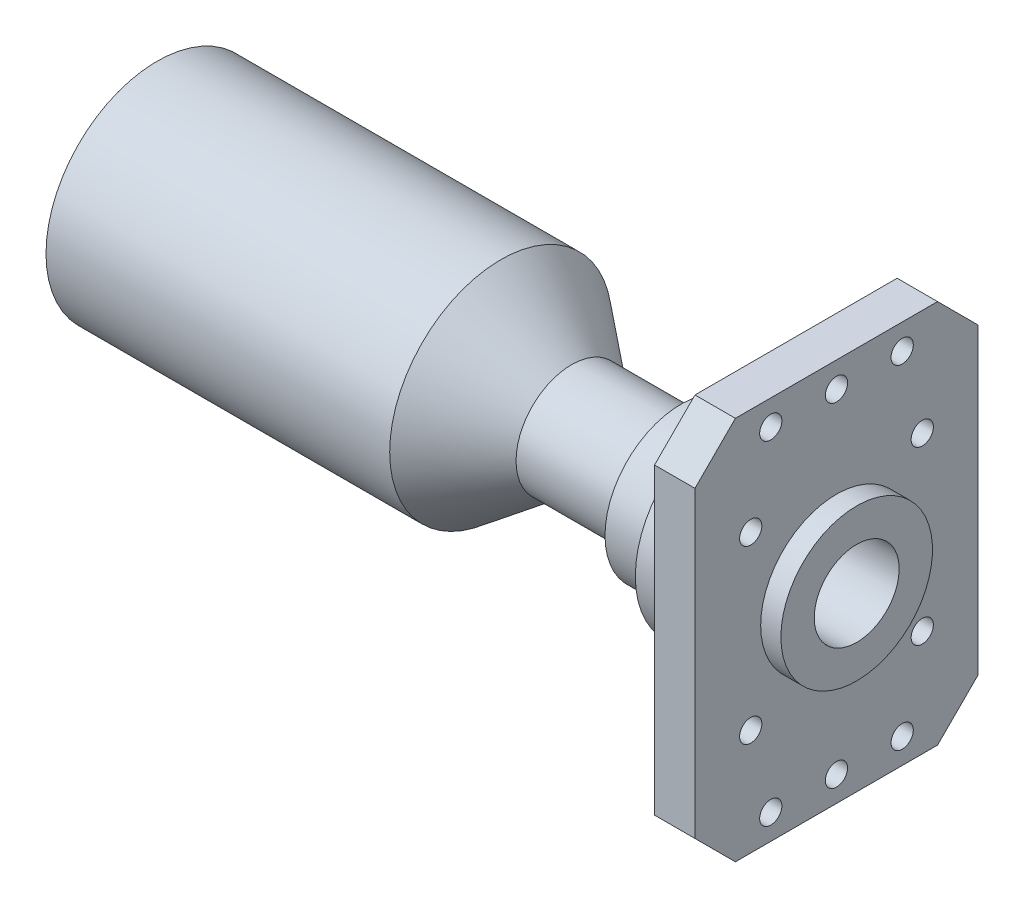
from build123d import *

# Parameters (mm, degrees)
CUT_EXTRUDE_1_REACH = 363.865
EXTRUDE_2_DEPTH     = 20
CUT_EXTRUDE_2_REACH = 358.119
SKETCH_4_R          = 5.5
SKETCH_5_R          = 55
SKETCH_5_R_2        = 42.5
EXTRUDE_3_DEPTH     = 170
CUT_EXTRUDE_START   = -175
SKETCH_8_R          = 35
CUT_EXTRUDE_3_DEPTH = 175
CUT_EXTRUDE_4_DEPTH = 47.5


with BuildPart() as part:
    # 草图1 → 旋转1 (revolve)
    with BuildSketch(Plane.XY, mode=Mode.PRIVATE) as revolve_1_sk:
        Polygon((106.222222222, -21), (56.222222222, -21), (56.222222222, -17.5), (-239.777777778, -17.5), (-239.777777778, -30), (-224.777777778, -30), (-224.777777778, -32.5), (-204.777777778, -32.5), (-204.777777778, -35), (-194.777777778, -35), (-187.277777778, -27.5), (19.222222222, -27.5), (19.222222222, -37.5), (44.222222222, -37.5), (44.222222222, -47.5), (64.222222222, -47.5), (76.222222222, -68.5), (76.222222222, -95), (96.222222222, -95), (96.222222222, -37.5), (106.222222222, -37.5), align=None)
    revolve(revolve_1_sk.sketch.rotate(Axis((-107.8, 0, 0), (1, 0, 0)), 270), axis=Axis((-107.8, 0, 0), (1, 0, 0)))

    # 草图2 → 切除-拉伸1 (cut, up to next)
    with BuildSketch(Plane(origin=(96.222222222, 0, 0), x_dir=(0, 0, -1), z_dir=(1, 0, 0)), mode=Mode.PRIVATE) as cut_extrude_1_sk1:
        with BuildLine():
            Line((70, -64.27376204), (70, 64.27376204))
            ThreePointArc((70, 64.27376204), (95.032186583, 0), (70, -64.27376204))
        make_face()
    cut_extrude_1_tool1 = extrude(cut_extrude_1_sk1.sketch, amount=-CUT_EXTRUDE_1_REACH, mode=Mode.PRIVATE) & part.part
    # 草图2 → 切除-拉伸1 (cut, up to next)
    with BuildSketch(Plane(origin=(96.222222222, 0, 0), x_dir=(0, 0, -1), z_dir=(1, 0, 0)), mode=Mode.PRIVATE) as cut_extrude_1_sk2:
        with BuildLine():
            Line((-70, -64.27376204), (-70, 64.27376204))
            ThreePointArc((-70, 64.27376204), (-95.032186583, 0), (-70, -64.27376204))
        make_face()
    cut_extrude_1_tool2 = extrude(cut_extrude_1_sk2.sketch, amount=-CUT_EXTRUDE_1_REACH, mode=Mode.PRIVATE) & part.part
    add(cut_extrude_1_tool1.solids().sort_by_distance((96.222222, 0, -80.135282))[0], mode=Mode.SUBTRACT)
    add(cut_extrude_1_tool2.solids().sort_by_distance((96.222222, 0, 80.135282))[0], mode=Mode.SUBTRACT)

    # 草图3 → 凸台-拉伸2 (add)
    with BuildSketch(Plane(origin=(96.222222222, 0, 0), x_dir=(0, 0, -1), z_dir=(1, 0, 0))):
        with BuildLine():
            Line((-70, 75), (-70, 64.226162893))
            ThreePointArc((-70, 64.226162893), (-38.232934266, 86.96690599), (0, 95))
            Line((0, 95), (-50, 95))
            Line((-50, 95), (-70, 75))
        make_face()
        with BuildLine():
            ThreePointArc((0, 95), (38.232934266, 86.96690599), (70, 64.226162893))
            Line((70, 64.226162893), (70, 75))
            Line((70, 75), (50, 95))
            Line((50, 95), (0, 95))
        make_face()
        with BuildLine():
            ThreePointArc((0, -95), (-38.232934266, -86.96690599), (-70, -64.226162893))
            Line((-70, -64.226162893), (-70, -75))
            Line((-70, -75), (-50, -95))
            Line((-50, -95), (0, -95))
        make_face()
        with BuildLine():
            Line((70, -75), (70, -64.226162893))
            ThreePointArc((70, -64.226162893), (38.232934266, -86.96690599), (0, -95))
            Line((0, -95), (50, -95))
            Line((50, -95), (70, -75))
        make_face()
    extrude(amount=-EXTRUDE_2_DEPTH)

    # 草图4 → 切除-拉伸2 (cut, up to next)
    with BuildSketch(Plane(origin=(96.222222222, 0, 0), x_dir=(0, 0, -1), z_dir=(1, 0, 0)), mode=Mode.PRIVATE) as cut_extrude_2_sk1:
        with Locations((42.426406871, 42.426406871)):
            Circle(SKETCH_4_R)
    cut_extrude_2_tool1 = extrude(cut_extrude_2_sk1.sketch, amount=-CUT_EXTRUDE_2_REACH, mode=Mode.PRIVATE) & part.part
    # 草图4 → 切除-拉伸2 (cut, up to next)
    with BuildSketch(Plane(origin=(96.222222222, 0, 0), x_dir=(0, 0, -1), z_dir=(1, 0, 0)), mode=Mode.PRIVATE) as cut_extrude_2_sk2:
        with Locations((42.426406871, -42.426406871)):
            Circle(SKETCH_4_R)
    cut_extrude_2_tool2 = extrude(cut_extrude_2_sk2.sketch, amount=-CUT_EXTRUDE_2_REACH, mode=Mode.PRIVATE) & part.part
    # 草图4 → 切除-拉伸2 (cut, up to next)
    with BuildSketch(Plane(origin=(96.222222222, 0, 0), x_dir=(0, 0, -1), z_dir=(1, 0, 0)), mode=Mode.PRIVATE) as cut_extrude_2_sk3:
        with Locations((-42.426406871, -42.426406871)):
            Circle(SKETCH_4_R)
    cut_extrude_2_tool3 = extrude(cut_extrude_2_sk3.sketch, amount=-CUT_EXTRUDE_2_REACH, mode=Mode.PRIVATE) & part.part
    # 草图4 → 切除-拉伸2 (cut, up to next)
    with BuildSketch(Plane(origin=(96.222222222, 0, 0), x_dir=(0, 0, -1), z_dir=(1, 0, 0)), mode=Mode.PRIVATE) as cut_extrude_2_sk4:
        with Locations((-42.426406871, 42.426406871)):
            Circle(SKETCH_4_R)
    cut_extrude_2_tool4 = extrude(cut_extrude_2_sk4.sketch, amount=-CUT_EXTRUDE_2_REACH, mode=Mode.PRIVATE) & part.part
    # 草图4 → 切除-拉伸2 (cut, up to next)
    with BuildSketch(Plane(origin=(96.222222222, 0, 0), x_dir=(0, 0, -1), z_dir=(1, 0, 0)), mode=Mode.PRIVATE) as cut_extrude_2_sk5:
        with Locations((0, 82.5)):
            Circle(SKETCH_4_R)
    cut_extrude_2_tool5 = extrude(cut_extrude_2_sk5.sketch, amount=-CUT_EXTRUDE_2_REACH, mode=Mode.PRIVATE) & part.part
    # 草图4 → 切除-拉伸2 (cut, up to next)
    with BuildSketch(Plane(origin=(96.222222222, 0, 0), x_dir=(0, 0, -1), z_dir=(1, 0, 0)), mode=Mode.PRIVATE) as cut_extrude_2_sk6:
        with Locations((-32.5, 82.5)):
            Circle(SKETCH_4_R)
    cut_extrude_2_tool6 = extrude(cut_extrude_2_sk6.sketch, amount=-CUT_EXTRUDE_2_REACH, mode=Mode.PRIVATE) & part.part
    # 草图4 → 切除-拉伸2 (cut, up to next)
    with BuildSketch(Plane(origin=(96.222222222, 0, 0), x_dir=(0, 0, -1), z_dir=(1, 0, 0)), mode=Mode.PRIVATE) as cut_extrude_2_sk7:
        with Locations((32.5, 82.5)):
            Circle(SKETCH_4_R)
    cut_extrude_2_tool7 = extrude(cut_extrude_2_sk7.sketch, amount=-CUT_EXTRUDE_2_REACH, mode=Mode.PRIVATE) & part.part
    # 草图4 → 切除-拉伸2 (cut, up to next)
    with BuildSketch(Plane(origin=(96.222222222, 0, 0), x_dir=(0, 0, -1), z_dir=(1, 0, 0)), mode=Mode.PRIVATE) as cut_extrude_2_sk8:
        with Locations(Location((32.5, -82.5, 0), (0, 0, 180))):
            Circle(SKETCH_4_R)
    cut_extrude_2_tool8 = extrude(cut_extrude_2_sk8.sketch, amount=-CUT_EXTRUDE_2_REACH, mode=Mode.PRIVATE) & part.part
    # 草图4 → 切除-拉伸2 (cut, up to next)
    with BuildSketch(Plane(origin=(96.222222222, 0, 0), x_dir=(0, 0, -1), z_dir=(1, 0, 0)), mode=Mode.PRIVATE) as cut_extrude_2_sk9:
        with Locations(Location((0, -82.5, 0), (0, 0, 180))):
            Circle(SKETCH_4_R)
    cut_extrude_2_tool9 = extrude(cut_extrude_2_sk9.sketch, amount=-CUT_EXTRUDE_2_REACH, mode=Mode.PRIVATE) & part.part
    # 草图4 → 切除-拉伸2 (cut, up to next)
    with BuildSketch(Plane(origin=(96.222222222, 0, 0), x_dir=(0, 0, -1), z_dir=(1, 0, 0)), mode=Mode.PRIVATE) as cut_extrude_2_sk10:
        with Locations(Location((-32.5, -82.5, 0), (0, 0, 180))):
            Circle(SKETCH_4_R)
    cut_extrude_2_tool10 = extrude(cut_extrude_2_sk10.sketch, amount=-CUT_EXTRUDE_2_REACH, mode=Mode.PRIVATE) & part.part
    add(cut_extrude_2_tool1.solids().sort_by_distance((96.222222, 42.426407, -42.426407))[0], mode=Mode.SUBTRACT)
    add(cut_extrude_2_tool2.solids().sort_by_distance((96.222222, -42.426407, -42.426407))[0], mode=Mode.SUBTRACT)
    add(cut_extrude_2_tool3.solids().sort_by_distance((96.222222, -42.426407, 42.426407))[0], mode=Mode.SUBTRACT)
    add(cut_extrude_2_tool4.solids().sort_by_distance((96.222222, 42.426407, 42.426407))[0], mode=Mode.SUBTRACT)
    add(cut_extrude_2_tool5.solids().sort_by_distance((96.222222, 82.5, 0))[0], mode=Mode.SUBTRACT)
    add(cut_extrude_2_tool6.solids().sort_by_distance((96.222222, 82.5, 32.5))[0], mode=Mode.SUBTRACT)
    add(cut_extrude_2_tool7.solids().sort_by_distance((96.222222, 82.5, -32.5))[0], mode=Mode.SUBTRACT)
    add(cut_extrude_2_tool8.solids().sort_by_distance((96.222222, -82.5, -32.5))[0], mode=Mode.SUBTRACT)
    add(cut_extrude_2_tool9.solids().sort_by_distance((96.222222, -82.5, 0))[0], mode=Mode.SUBTRACT)
    add(cut_extrude_2_tool10.solids().sort_by_distance((96.222222, -82.5, 32.5))[0], mode=Mode.SUBTRACT)



with BuildPart() as body_2:
    # 草图5 → 凸台-拉伸3 (new body)
    with BuildSketch(Plane.ZY.offset(239.777777778)):
        Circle(SKETCH_5_R)
        Circle(SKETCH_5_R_2, mode=Mode.SUBTRACT)
    extrude(amount=-EXTRUDE_3_DEPTH)


with BuildPart() as part_1:
    add(part.part)

    add(body_2.part)  # 旋转2 merges body 2
    # 草图7 → 旋转2 (revolve)
    with BuildSketch(Plane.XY, mode=Mode.PRIVATE) as revolve_2_sk:
        Polygon((-69.777777778, 55), (-69.777777778, 27.5), (-34.777777778, 27.5), align=None)
    revolve(revolve_2_sk.sketch.rotate(Axis((-69.777777778, 0, 0), (-1, 0, 0)), 270), axis=Axis((-69.777777778, 0, 0), (-1, 0, 0)))

    # 草图8 → 切除-拉伸3 (cut)
    with BuildSketch(Plane.ZY.offset(239.777777778).offset(CUT_EXTRUDE_START)):
        Circle(SKETCH_8_R)
    extrude(amount=CUT_EXTRUDE_3_DEPTH, mode=Mode.SUBTRACT)

    # 草图9 → 切除-拉伸4 (cut, symmetric)
    with BuildSketch(Plane.XY):
        with BuildLine():
            Line((-224.777777778, 11), (-89.777777778, 11))
            ThreePointArc((-89.777777778, 11), (-78.777777778, 0), (-89.777777778, -11))
            Line((-89.777777778, -11), (-224.777777778, -11))
            ThreePointArc((-224.777777778, -11), (-235.777777778, 0), (-224.777777778, 11))
        make_face()
    extrude(amount=CUT_EXTRUDE_4_DEPTH, both=True, mode=Mode.SUBTRACT)


solid = part_1.part
